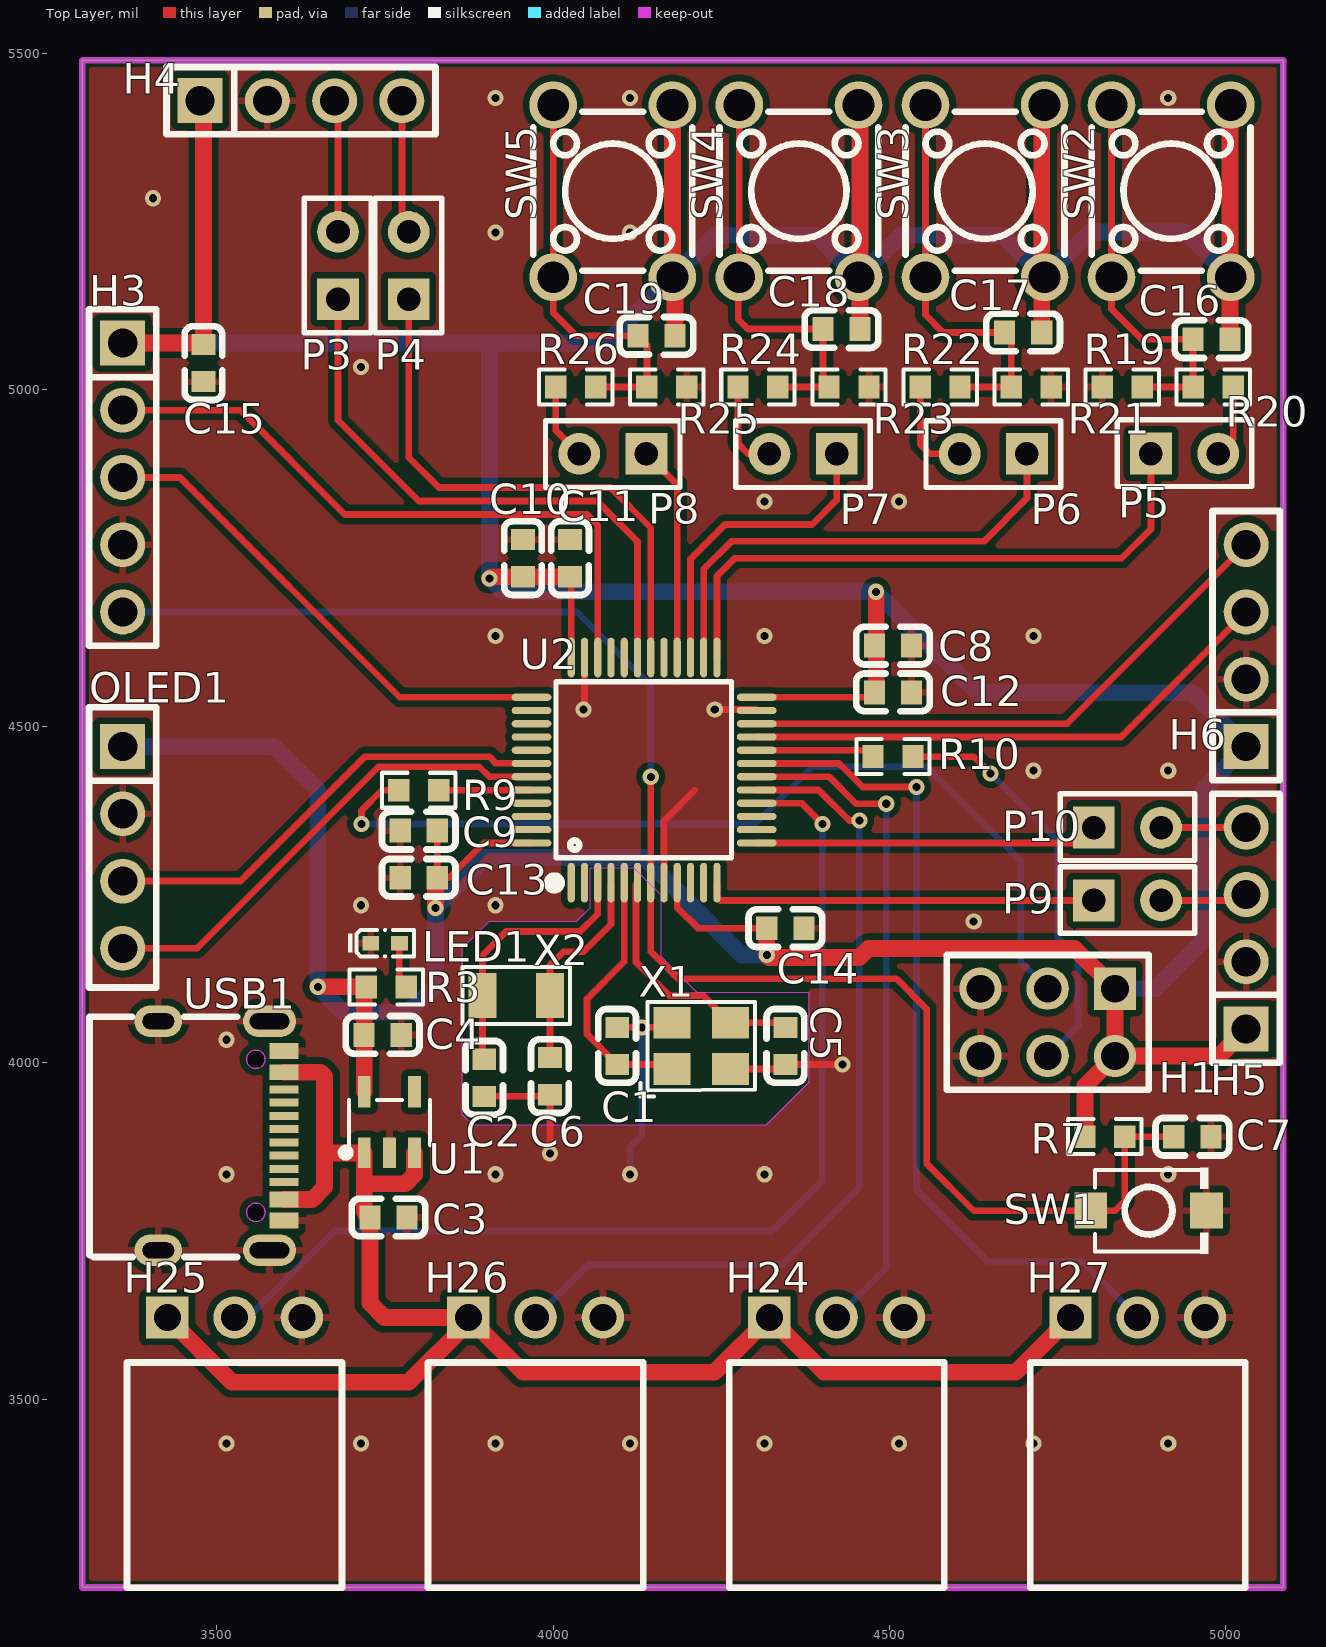
[diagram p0: Top Layer view]
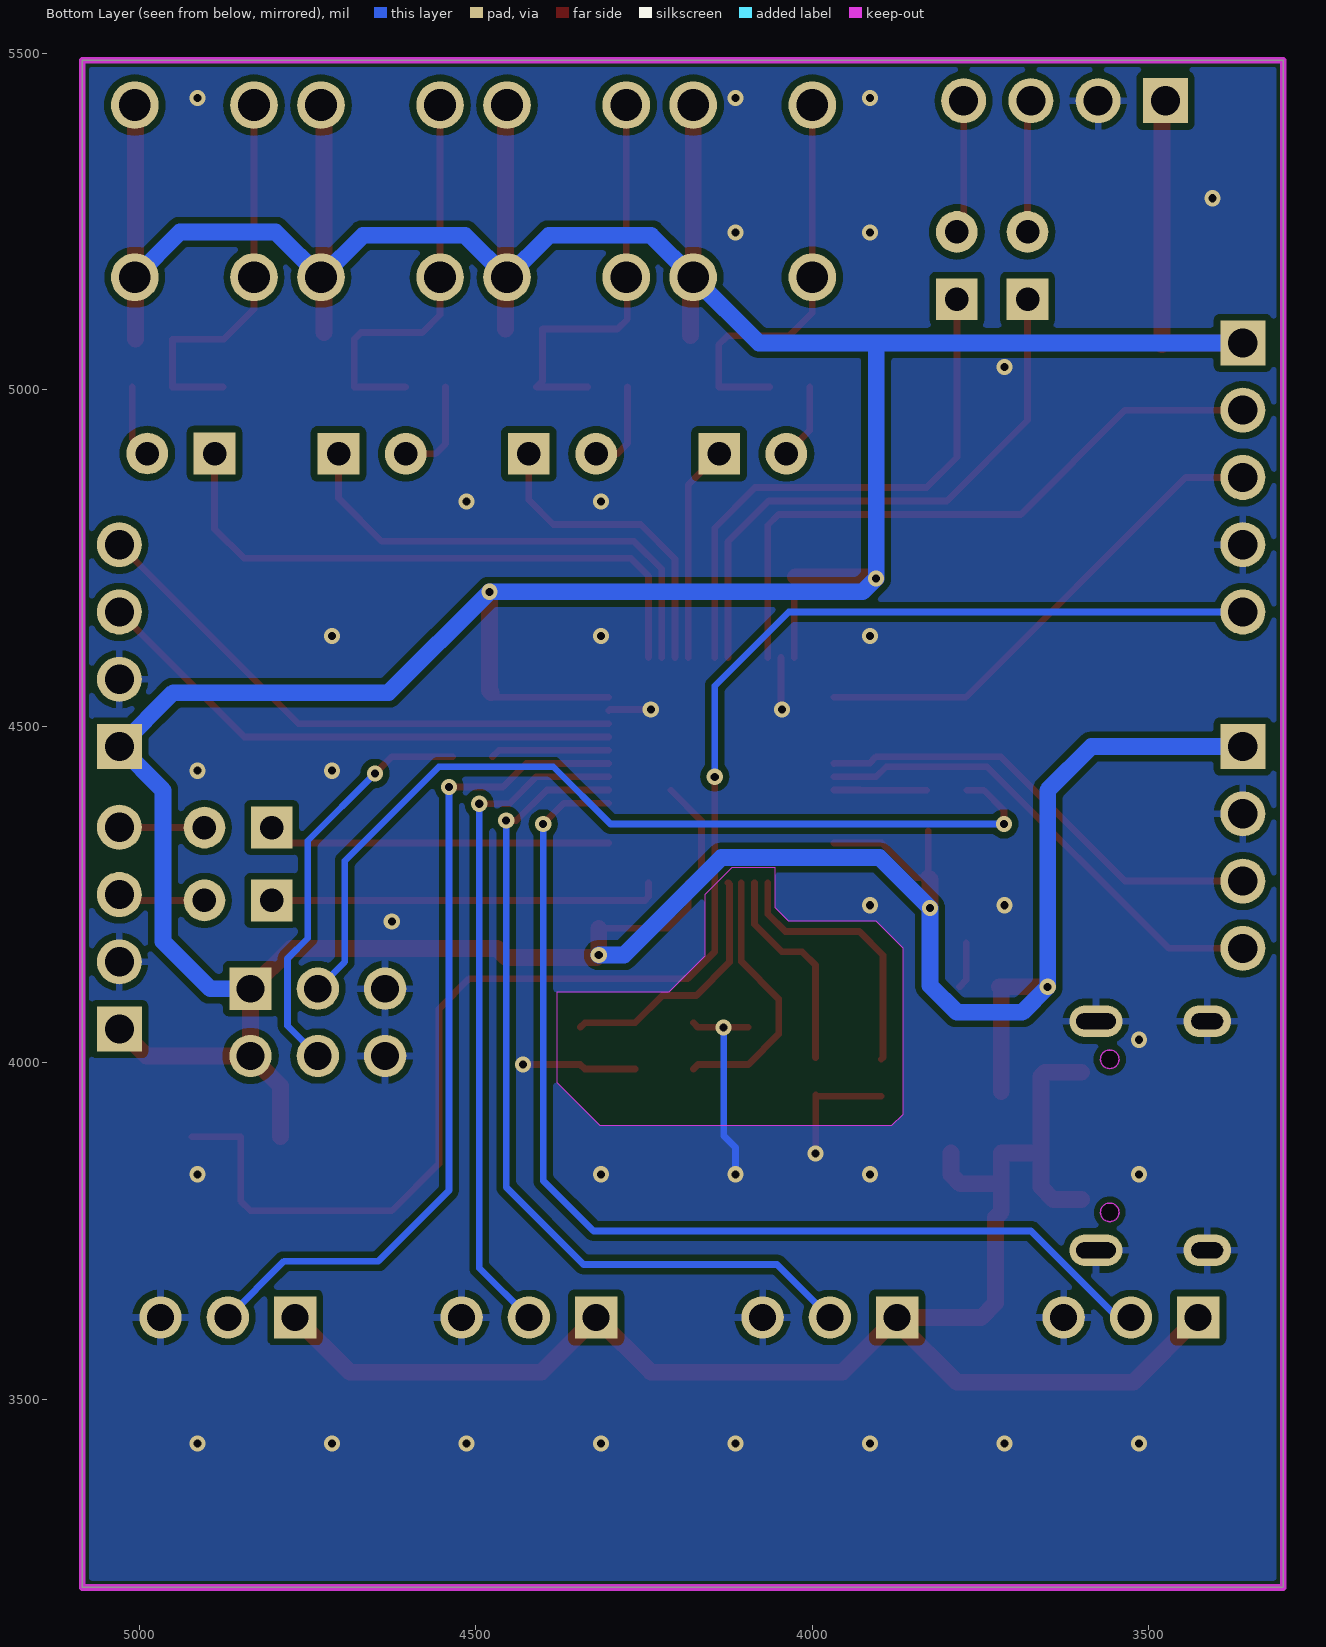
[diagram p1: Bottom Layer view, seen from below]
# Altium PCB MISC61607.pcbdoc
Units mil, origin at the board's own origin, x right, y up, seen from the top; angles counter-clockwise.
Board outline 1785 x 2270 mil, 2 copper layers (Top Layer, Bottom Layer), stack 62.206 mil thick; 60 components, 58 nets, 212 pads, 48 vias.

## Layer stack, top to bottom
Top Solder Mask Layer: solder mask 0.394, Dk 3.3
Top Layer: signal copper 1.379
Dielectric1: surface 59.449, FR4, Dk 4.5
Bottom Layer: signal copper 1.378
Bottom Solder Mask Layer: solder mask 0.394, Dk 3.3

## Board outline
3300,5490 3300,3220 5085,3220 5085,5490

## Design rules (kind name [scope] priority, off if disabled: settings)
BoardOutlineClearance copperThickness2oz_1 [All] p2 off: genericclearance=7.99 ignorepadtopadclearanceinfootprint=FALSE except(0: Arc-SplitContinuation Track-SplitContinuation SMDPad-SplitContinuation THPad-SplitContinuation Via-SplitContinuation Fill-SplitContinuation Region-SplitContinuation Poly-SplitContinuation Text-SplitContinuation Hole-SplitContinuation; 5.98: Arc-CutoutEdge SMDPad-CutoutEdge THPad-CutoutEdge Via-CutoutEdge Fill-CutoutEdge Region-CutoutEdge Text-CutoutEdge; 6.93: Hole-OutlineEdge Hole-CutoutEdge; 10: Poly-OutlineEdge Poly-CutoutEdge; 11.81: Arc-OutlineEdge Track-OutlineEdge SMDPad-OutlineEdge THPad-OutlineEdge Via-OutlineEdge Fill-OutlineEdge Region-OutlineEdge Text-OutlineEdge Track-CutoutEdge)
BoardOutlineClearance copperThickness1oz_1 [All] p4: genericclearance=4.02 ignorepadtopadclearanceinfootprint=FALSE except(0: Arc-SplitContinuation Track-SplitContinuation SMDPad-SplitContinuation THPad-SplitContinuation Via-SplitContinuation Fill-SplitContinuation Region-SplitContinuation Poly-SplitContinuation Text-SplitContinuation Hole-SplitContinuation; 6: SMDPad-CutoutEdge THPad-CutoutEdge Via-CutoutEdge Fill-CutoutEdge Region-CutoutEdge Text-CutoutEdge; 6.93: Hole-OutlineEdge Hole-CutoutEdge; 10: Poly-OutlineEdge Poly-CutoutEdge; 11.8: Arc-OutlineEdge Track-OutlineEdge SMDPad-OutlineEdge THPad-OutlineEdge Via-OutlineEdge Fill-OutlineEdge Region-OutlineEdge Text-OutlineEdge; 11.81: Arc-CutoutEdge Track-CutoutEdge)
Clearance copperThickness2oz [All] p1 off: gap=7.99 ignorepadtopadclearanceinfootprint=FALSE except(5.98: SMDPad-Track SMDPad-SMDPad THPad-Track SMDPad-THPad THPad-THPad Track-Via SMDPad-Via THPad-Via Via-Via Fill-Track Region-Track Fill-SMDPad Region-SMDPad Fill-THPad Region-THPad Fill-Via Region-Via Fill-Fill Fill-Region Region-Region Arc-Track Arc-SMDPad Arc-THPad Arc-Via Fill-Arc Region-Arc Arc-Arc Text-Track SMDPad-Text Text-THPad Text-Via Fill-Text Region-Text Arc-Text Text-Text; 6.93: Hole-Track Hole-SMDPad Hole-THPad Hole-Via Fill-Hole Region-Hole Hole-Arc Hole-Text; 10: Poly-Track Poly-SMDPad Poly-THPad Poly-Via Poly-Fill Poly-Region Poly-Poly Poly-Arc Poly-Text Poly-Hole)
Clearance copperThickness1oz [All] p3: gap=4.02 ignorepadtopadclearanceinfootprint=FALSE except(5.98: SMDPad-Track SMDPad-SMDPad THPad-Track SMDPad-THPad THPad-THPad Track-Via SMDPad-Via THPad-Via Via-Via Fill-Track Region-Track Fill-SMDPad Region-SMDPad Fill-THPad Region-THPad Fill-Via Region-Via Fill-Fill Fill-Region Region-Region; 6: Arc-Track Arc-SMDPad Arc-THPad Arc-Via Fill-Arc Region-Arc Arc-Arc Text-Track SMDPad-Text Text-THPad Text-Via Fill-Text Region-Text Arc-Text Text-Text; 6.93: Hole-Track Hole-SMDPad Hole-THPad Hole-Via Fill-Hole Region-Hole Hole-Arc Hole-Text; 10: Poly-Track Poly-SMDPad Poly-THPad Poly-Via Poly-Fill Poly-Region Poly-Poly Poly-Arc Poly-Text Poly-Hole)
DiffPairsRouting differentialPair [All] p1: maxlimit=6 minlimit=6 mostfreqgap=6 toplayer_minwidth=5 toplayer_prefwidth=10 toplayer_maxwidth=100 toplayer_mingap=6 toplayer_prefgap=6 toplayer_maxgap=6 bottomlayer_minwidth=5 bottomlayer_prefwidth=10 bottomlayer_maxwidth=100 bottomlayer_mingap=6 bottomlayer_prefgap=6 bottomlayer_maxgap=6 maxuncoupledlength=10
HoleToHoleClearance otherClearance [All] p1: gap=11.81 allowstackedmicrovias=TRUE
Length netLength [All] p1: minlimit=0 maxlimit=0
MatchedLengths netLengthTolerance [All] p1: tolerance=1000
PasteMaskExpansion pasteMaskExpansion [All] p1: expansion=0
PlaneConnect innerPlane [All] p1: planeconnectstyle=Relief reliefexpansion=20 reliefentries=4 reliefconductorwidth=10 reliefairgap=10
PolygonConnect copperRegion [(InNet('GND'))] p1: connectstyle=Relief reliefconductorwidth=10 reliefentries=4 polygonreliefangle="90 Angle" airgapwidth=10 via.connectstyle=Relief via.reliefconductorwidth=10 via.reliefentries=4 via.polygonreliefangle="90 Angle" via.airgapwidth=10
RoutingVias viaSize [All] p1: holewidth=12.01 width=24.02 viastyle="Through Hole" minholewidth=11.81 minwidth=19.68 maxholewidth=248.03 maxwidth=393.7
SolderMaskExpansion solderMaskExpansion [IsVia] p1: expansion=-1000 istentingtop=TRUE
SolderMaskExpansion solderMaskExpansion [All] p2: expansion=2 istentingtop=FALSE
Width copperThickness2oz_2 [All] p1 off: maxlimit=100 minlimit=8 preferedwidth=10
Width copperThickness1oz_2 [All] p2: maxlimit=100 minlimit=5 preferedwidth=10

## Components (designator, comment, footprint, x,y, rotation, side; value= is the part's Value field where it differs from the comment)
C1 "18pF" C0603 4095,4025 r90 top
C2 "10pF" C0603 3897.44,3977.56 r90 top
C3 "1uF" C0603 3755,3770 r180 top
C4 "1uF" C0603 3746.42,4041.36 r180 top
C5 "18pF" C0603 4345,4025 r270 top
C6 "10pF" C0603 3995,3980 r90 top
C7 "1uF" C0603 4950,3890 r0 top
C8 "4.7uF" C0603 4505,4620 r180 top
C9 "100nF" C0603 3800,4345 r180 top
C10 "100nF" C0603 3955,4750 r90 top
C11 "100nF" C0603 4025,4750 r270 top
C12 "100nF" C0603 4505,4550.53 r180 top
C13 "100nF" C0603 3800,4275 r0 top
C14 "100nF" C0603 4345,4200 r180 top
C15 "100nF" C0603 3480,5040 r90 top
C16 "100nF" C0603 4978.47,5075.55 r0 top
C17 "100nF" C0603 4698.47,5085.55 r0 top
C18 "100nF" C0603 4428.47,5090.55 r0 top
C19 "100nF" C0603 4153.47,5080.55 r0 top
H1 "" HDR-TH_6P-P2.54-V-R2-C3-S2.54_A2541WV-2X3P 4735,4060 r180 top
H3 "PZ254V-11-05P" HDR-TH_5P-P2.54-V-M 3360,4870 r270 top
H4 "PZ254V-11-04P" HDR-TH_4P-P2.54-V-M 3625,5430 r0 top
H5 "PZ254V-11-04P" HDR-TH_4P-P2.54-V-M 5030,4200 r90 top
H6 "PZ254V-11-04P" HDR-TH_4P-P2.54-V-M 5030,4620 r90 top
H24 "HC-PM254-8.5H-1x3PW-02A" HDR-TH_3P-P2.54_HC-PM254-8.5H-1X3PW 4421.3,3621.27 r0 top
H25 "HC-PM254-8.5H-1x3PW-02A" HDR-TH_3P-P2.54_HC-PM254-8.5H-1X3PW 3526.27,3621.27 r0 top
H26 "HC-PM254-8.5H-1x3PW-02A" HDR-TH_3P-P2.54_HC-PM254-8.5H-1X3PW 3973.78,3621.27 r0 top
H27 "HC-PM254-8.5H-1x3PW-02A" HDR-TH_3P-P2.54_HC-PM254-8.5H-1X3PW 4868.81,3621.27 r0 top
LED1 "" LED_0402 3749.97,4177.82 r0 top
OLED1 "2.54-1*4P female" HDR-TH_4P-P2.54-V-F 3360,4320 r270 top
P3 "Jumper pin header" 2P排针 3680,5185 r90 top
P4 "Jumper pin header" 2P排针 3785,5185 r90 top
P5 "Jumper pin header" 2P排针 4938.47,4905.55 r0 top
P6 "Jumper pin header" 2P排针 4654.16,4905.08 r180 top
P7 "Jumper pin header" 2P排针 4371.31,4905.08 r180 top
P8 "Jumper pin header" 2P排针 4088.47,4905.08 r180 top
P9 "Jumper pin header" 2P排针 4853.54,4241.28 r0 top
P10 "Jumper pin header" 2P排针 4853.54,4349.54 r0 top
R3 "1kΩ" R0603 3751.58,4112.82 r0 top
R7 "10kΩ" R0603 4820,3890 r180 top
R9 "10kΩ" R0603 3800,4405 r180 top
R10 "10kΩ" R0603 4505,4455 r180 top
R19 "4.7kΩ" R0603 4845.78,5004.36 r0 top
R20 "1kΩ" R0603 4981.17,5004.36 r180 top
R21 "4.7kΩ" R0603 4710.4,5004.36 r180 top
R22 "1kΩ" R0603 4575.01,5004.36 r0 top
R23 "4.7kΩ" R0603 4439.62,5004.36 r180 top
R24 "1kΩ" R0603 4304.24,5004.36 r0 top
R25 "4.7kΩ" R0603 4168.85,5004.36 r180 top
R26 "1kΩ" R0603 4033.47,5004.36 r0 top
SW1 "TS-1088-AR02016" SW-SMD_L3.9-W3.0-P4.45 4885,3780 r0 top
SW2 "TS665CJ" SW-TH_4P-L6.0-W6.0-P4.50-LS6.5 4918.47,5295.55 r90 top
SW3 "TS665CJ" SW-TH_4P-L6.0-W6.0-P4.50-LS6.5 4641.8,5295.55 r90 top
SW4 "TS665CJ" SW-TH_4P-L6.0-W6.0-P4.50-LS6.5 4365.13,5295.55 r90 top
SW5 "TS665CJ" SW-TH_4P-L6.0-W6.0-P4.50-LS6.5 4088.47,5295.55 r90 top
U1 "ME6211C33M5G-N" SOT-23-5_L3.0-W1.7-P0.95-LS2.8-BL 3756.42,3911.36 r0 top
U2 "STM32F103C8T6" LQFP-48_L7.0-W7.0-P0.50-LS9.0-BL 4135,4435 r0 top
USB1 "TYPE-C 16PIN 2MD(073)" USB-C-SMD_TYPE-C-6PIN-2MD-073 3506.42,3891.36 r270 top
X1 "8MHz" OSC-SMD_4P-L3.2-W2.5-BL 4220,4025 r0 top
X2 "32.768kHz" CRYSTAL-SMD_L3.2-W1.5-1 3945,4100 r180 top

## Footprints (in the part's own frame and the unit in brackets; to place one, negate y for a bottom-side part, rotate by r counter-clockwise, add the part's x,y. Pads: shape width x height; smd on the part's side, far side on the other; paste and mask are expansions set on the pad)
2P排针 [mil]
  rect 62x62 hole 35: 1(-50,0)
  round 62 hole 35: 2(50,0)
  silkscreen extent -100,-49 100,50
C0603 [mm]
  rect 0.8x0.9 smd: 1(-0.7,0) 2(0.7,0)
  silkscreen extent -1.39,-0.71 1.39,0.71
CRYSTAL-SMD_L3.2-W1.5-1 [mm]
  rect 1.05x1.7 smd: 1(-1.275,0) 2(1.275,0)
  silkscreen extent -2.03,-1.08 2.03,1.08
HDR-TH_3P-P2.54_HC-PM254-8.5H-1X3PW [mm]
  rect 1.6x1.6 hole 1.02: 1(-2.54,0)
  round 1.6 hole 1.02: 2(0,0) 3(2.54,0)
  silkscreen extent -4.06,-10.2 4.06,-1.7
HDR-TH_4P-P2.54-V-F [mm]
  rect 1.7x1.7 hole 1.1: 1(-3.81,0)
  round 1.7 hole 1.1: 2(-1.27,0) 3(1.27,0) 4(3.81,0)
  silkscreen extent -5.29,-1.27 5.29,1.27
HDR-TH_4P-P2.54-V-M [mm]
  rect 1.7x1.7 hole 1.1: 1(-3.81,0)
  round 1.7 hole 1.1: 2(-1.27,0) 3(1.27,0) 4(3.81,0)
  silkscreen extent -5.08,-1.27 5.08,1.27
HDR-TH_5P-P2.54-V-M [mm]
  rect 1.7x1.7 hole 1.1: 1(-5.08,0)
  round 1.7 hole 1.1: 2(-2.54,0) 3(0,0) 4(2.54,0) 5(5.08,0)
  silkscreen extent -6.35,-1.27 6.35,1.27
HDR-TH_6P-P2.54-V-R2-C3-S2.54_A2541WV-2X3P [mm]
  rect 1.6x1.6 hole 1.05: 1(-2.54,-1.27)
  round 1.6 hole 1.05: 2(-2.54,1.27) 3(0,-1.27) 4(0,1.27) 5(2.54,-1.27) 6(2.54,1.27)
  silkscreen extent -3.81,-2.54 3.81,2.54
LED_0402 [mil]
  rect 25.1x21.3 smd paste-3937.01 mask+2: 1(-21.2,0) 2(21.2,0)
  silkscreen extent -55,-21 43,21
LQFP-48_L7.0-W7.0-P0.50-LS9.0-BL [mm]
  oval 0.27x1.5 smd paste+0 mask+0.05: 1(-2.75,-4.25) 2(-2.25,-4.25) 3(-1.75,-4.25) 4(-1.25,-4.25) 5(-0.75,-4.25) 6(-0.25,-4.25) 7(0.25,-4.25) 8(0.75,-4.25) 9(1.25,-4.25) 10(1.75,-4.25) 11(2.25,-4.25) 12(2.75,-4.25) 25(2.75,4.25) 26(2.25,4.25) 27(1.75,4.25) 28(1.25,4.25) 29(0.75,4.25) 30(0.25,4.25) 31(-0.25,4.25) 32(-0.75,4.25) 33(-1.25,4.25) 34(-1.75,4.25) 35(-2.25,4.25) 36(-2.75,4.25)
  oval 1.5x0.27 smd paste+0 mask+0.05: 13(4.25,-2.75) 14(4.25,-2.25) 15(4.25,-1.75) 16(4.25,-1.25) 17(4.25,-0.75) 18(4.25,-0.25) 19(4.25,0.25) 20(4.25,0.75) 21(4.25,1.25) 22(4.25,1.75) 23(4.25,2.25) 24(4.25,2.75) 37(-4.25,2.75) 38(-4.25,2.25) 39(-4.25,1.75) 40(-4.25,1.25) 41(-4.25,0.75) 42(-4.25,0.25) 43(-4.25,-0.25) 44(-4.25,-0.75) 45(-4.25,-1.25) 46(-4.25,-1.75) 47(-4.25,-2.25) 48(-4.25,-2.75)
  silkscreen extent -3.59,-4.46 3.3,3.34
OSC-SMD_4P-L3.2-W2.5-BL [mm]
  rect 1.4x1.2 smd: 1(-1.1,-0.875) 2(1.1,-0.875) 3(1.1,0.875) 4(-1.1,0.875)
  silkscreen extent -2.29,-1.9 2.03,1.65
R0603 [mil]
  rect 31.75x34.02 smd paste-3937.01 mask+2: 1(-29.66,0) 2(29.66,0)
  silkscreen extent -55,-26 55,26
SOT-23-5_L3.0-W1.7-P0.95-LS2.8-BL [mm]
  rect 0.49x1.157 smd: 1(-0.95,-1.154) 2(0,-1.154) 3(0.95,-1.154)
  rect 0.49x1.175 smd: 4(0.95,1.154) 5(-0.95,1.154)
  silkscreen extent -1.8,-1.29 1.53,0.85
SW-SMD_L3.9-W3.0-P4.45 [mm]
  rect 1.23x1.36 smd: 1(-2.185,0) 2(2.185,0)
  silkscreen extent -2.03,-1.62 2.25,1.62
SW-TH_4P-L6.0-W6.0-P4.50-LS6.5 [mm]
  round 1.8 hole 1.2: 1(-3.25,2.25) 2(3.25,2.25) 3(-3.25,-2.25) 4(3.25,-2.25)
  silkscreen extent -3,-3 3,3
USB-C-SMD_TYPE-C-6PIN-2MD-073 [mm]
  rect 0.6x1.1 smd paste-100 mask+0.05: 1(-3.2,2.375) 2(-2.4,2.375) 11(2.4,2.375) 12(3.2,2.375)
  rect 0.3x1.1 smd paste-100 mask+0.05: 3(-1.75,2.375) 4(-1.25,2.375) 5(-0.75,2.375) 6(-0.25,2.375) 7(0.25,2.375) 8(0.75,2.375) 9(1.25,2.375) 10(1.75,2.375)
  oval 1.2x2 hole 0.6 slot 1.5 at 90 deg paste+0 mask+0.05: 13(-4.325,1.825) 14(4.325,1.825)
  oval 1.2x1.8 hole 0.6 slot 1.2 at 90 deg paste+0 mask+0.05: 13(-4.325,-2.375) 14(4.325,-2.375)
  Board Outline Layer circle w0.003: c-2.89,1.305 r0.35
  Board Outline Layer circle w0.003: c2.89,1.305 r0.35
  Board Outline Layer region: -2.89,1.655 -2.738,1.62 -2.616,1.523 -2.549,1.383 -2.549,1.227 -2.616,1.087 -2.738,0.99 -2.89,0.955 -2.89,0.955 -3.042,0.99 -3.164,1.087 -3.231,1.227 -3.231,1.383 -3.164,1.523 -3.042,1.62 -2.89,1.655
  Board Outline Layer region: -2.89,1.655 -2.812,1.646 -2.738,1.62 -2.672,1.579 -2.616,1.523 -2.575,1.457 -2.549,1.383 -2.54,1.305 -2.549,1.227 -2.575,1.153 -2.616,1.087 -2.672,1.031 -2.738,0.99 -2.812,0.964 -2.89,0.955 -2.968,0.964 -3.042,0.99 -3.108,1.031 -3.164,1.087 -3.205,1.153 -3.231,1.227 -3.24,1.305 -3.231,1.383 -3.205,1.457 -3.164,1.523 -3.108,1.579 -3.042,1.62 -2.968,1.646
  Board Outline Layer region: 2.89,1.655 3.042,1.62 3.164,1.523 3.231,1.383 3.231,1.227 3.164,1.087 3.042,0.99 2.89,0.955 2.89,0.955 2.738,0.99 2.616,1.087 2.549,1.227 2.549,1.383 2.616,1.523 2.738,1.62 2.89,1.655
  Board Outline Layer region: 2.89,1.655 2.968,1.646 3.042,1.62 3.108,1.579 3.164,1.523 3.205,1.457 3.231,1.383 3.24,1.305 3.231,1.227 3.205,1.153 3.164,1.087 3.108,1.031 3.042,0.99 2.968,0.964 2.89,0.955 2.812,0.964 2.738,0.99 2.672,1.031 2.616,1.087 2.575,1.153 2.549,1.227 2.54,1.305 2.549,1.383 2.575,1.457 2.616,1.523 2.672,1.579 2.738,1.62 2.812,1.646
  Multi-Layer board cut-out: -2.89,1.655 -2.738,1.62 -2.616,1.523 -2.549,1.383 -2.549,1.227 -2.616,1.087 -2.738,0.99 -2.89,0.955 -2.89,0.955 -3.042,0.99 -3.164,1.087 -3.231,1.227 -3.231,1.383 -3.164,1.523 -3.042,1.62 -2.89,1.655
  Multi-Layer board cut-out: 2.89,1.655 3.042,1.62 3.164,1.523 3.231,1.383 3.231,1.227 3.164,1.087 3.042,0.99 2.89,0.955 2.89,0.955 2.738,0.99 2.616,1.087 2.549,1.227 2.549,1.383 2.616,1.523 2.738,1.62 2.89,1.655
  silkscreen extent -4.5,-4.97 4.57,0.6

## Via types
v1: diameter 24.02, hole 12, Top Layer to Bottom Layer, 48 vias

## Nets (pads, with @x,y where several pads share a name; then routed paths per layer and width w, separated by ;. In a path a pad name is that pad's centre, name@x,y a point inside that pad or via, vN(x,y) a via of type N, cw(c..) or ccw(c..) an arc to the next point about the centre after c; other vN are vias at no path point)
$1N5475: LED1.2 R3.2 | length 69.2
  Top Layer w10: LED1.2 3771.17,4122.88 R3.2
$1N5490: H1.4 R10.1 | length 618.2
  Top Layer w10: R10.1 4625,4455 v1(4650,4430)
  Bottom Layer w10: v1(4650,4430) 4750,4330 4750,4185 4780,4155 4780,4055 H1.4
$1N5491: H1.3 R9.2 | length 1367.5
  Top Layer w10: v1(3715,4355) 3715,4375 3745,4405 R9.2
  Bottom Layer w10: v1(3715,4355) 4300,4355 4385,4440 4555,4440 4695,4300 4695,4150 H1.3
$1N5608: H4.3 P3.2 | length 197.1
  Top Layer w10: H4.3 3680,5425 P3.2
$1N5609: H4.4 P4.2 | length 199.1
  Top Layer w10: H4.4 3775,5245 P4.2
$1N5610: C19.1 R25.2 R26.2 SW5.1 SW5.2 | length 606.5
  Top Layer w10: SW5.2 SW5.1 3999.89,5115.11 4034.45,5080.55 C19.1 4139.19,5067.26 R25.2 R26.2
$1N5614: P6.2 R22.1 | length 149.3
  Top Layer w10: R22.1 4545.35,4920 4560.26,4905.09 P6.2
$1N5615: P8.2 R26.1 | length 113.6
  Top Layer w10: R26.1 4003.81,4939.74 P8.2
$1N5618: C17.1 R21.2 R22.2 SW3.1 SW3.2 | length 601.6
  Top Layer w10: SW3.2 SW3.1 4553.22,5111.78 4579.45,5085.55 C17.1 4680.74,5075.72 R21.2 R22.2
$1N5623: P7.2 R24.1 | length 137
  Top Layer w10: R24.1 4274.58,4920.42 4289.91,4905.09 P7.2
$1N5624: C18.1 R23.2 R24.2 SW4.1 SW4.2 | length 617
  Top Layer w10: SW4.2@4276.55,5423.5 4276.55,5167.6 4275,5166.04 4275,5105 4289.45,5090.55 C18.1 4400.91,5013.42 R23.2 R24.2
$1N5632: C16.1 R19.2 R20.2 SW2.1 SW2.2 | length 590.4
  Top Layer w10: SW2.2 SW2.1 4829.89,5120.11 4874.45,5075.55 C16.1 4950.91,5004.96 R20.2 R19.2
$1N5633: P5.2 R20.1 | length 108.1
  Top Layer w10: P5.2 5010.83,4927.9 R20.1
$1N5806: H5.3 P9.2 | length 130.1
  Top Layer w10: P9.2 5021.28,4241.28 H5.3
$1N5807: H5.4 P10.2 | length 126.7
  Top Layer w10: P10.2 5029.53,4349.53 H5.4
+5V: C3.2 H24.1 H25.1 H26.1 H27.1 U1.1 U1.3 USB1.2 USB1.11 | length 2410.4
  Top Layer w25: H25.1 3522.54,3525 3785,3525 3873.78,3613.78 H26.1 ; USB1.11 3641.86,3796.86 3660,3815 3660,3865.94 ; USB1.2 3654.16,3985.84 3660,3980 3660,3865.94 ; U1.3 3793.82,3833.82 3780,3820 3719.74,3820 3719.02,3819.28 ; H27.1 4687.54,3540 4402.57,3540 H24.1 4240.03,3540 3955.05,3540 H26.1 ; 3660,3865.94 U1.1 3719.02,3819.28 ; 3719.02,3819.28 3719.02,3778.42 C3.2 3727.44,3642.56 3748.73,3621.27 H26.1
BOOT0: R9.1 U2.44 | length 138.2
  Top Layer w10: R9.1 3929.06,4405 3929.53,4405.47 U2.44
BOOT1: R10.2 U2.20 | length 177
  Top Layer w10: U2.20 4465.81,4464.53 R10.2
GND: C1.2 C2.1 C3.1 C4.1 C5.2 C6.1 C7.2 C8.1 C9.2 C10.2 C11.1 C12.1 C13.1 C14.1 C15.1 H1.5 H1.6 H3.4 H4.2 H5.2 H6.2 H24.3 H25.3 H26.3 H27.3 LED1.1 OLED1.2 R19.1 R21.1 R23.1 R25.1 SW1.2 U1.2 U2.8 U2.23 U2.35 USB1.1 USB1.12 USB1.13 USB1.14 X1.2 X1.4 | length 962.8
  Top Layer w10: C2.1 3992.56,3950 C6.1 v1(3995,3865) ; v1(4045,4525) 4046.42,4526.42 U2.35 ; C1.2 v1(4131.72,4052.56) 4169.8,4052.56 X1.4 ; U2.8 4164.53,4359.53 4210,4405 ; v1(4240,4525) 4300.9,4525 U2.23 ; X1.2 4338.11,3990.55 C5.2 v1(4430,3997.44)
  Bottom Layer w10: v1(4114.1,3834.1) 4114.1,3874.1 4131.72,3891.72 v1(4131.72,4052.56)
  other v1: 3514.1,3434.1 3714.1,3434.1 3914.1,3434.1 4114.1,3434.1 4314.1,3434.1 4514.1,3434.1 4714.1,3434.1 4914.1,3434.1 3514.1,3834.1 3914.1,3834.1 4314.1,3834.1 4914.1,3834.1 3514.1,4034.1 4625,4210 3714.1,4234.1 3914.1,4234.1 4714.1,4434.1 4914.1,4434.1 3914.1,4634.1 4314.1,4634.1 4714.1,4634.1 4314.1,4834.1 4514.1,4834.1 3714.1,5034.1 3914.1,5234.1 4114.1,5234.1 3405,5285 3914.1,5434.1 4114.1,5434.1 4914.1,5434.1
NRST: C7.1 H3.5 R7.1 SW1.1 U2.7 | length 2398.8
  Top Layer w10: v1(4145,4425) 4145,4267.84 U2.7 4144.84,4165.16 4185,4125 4510,4125 4555,4080 4555,3850 4625,3780 SW1.1 4835,3780 4849.66,3794.66 R7.1 C7.1
  Bottom Layer w10: H3.5 4035,4670 4145,4560 v1(4145,4425)
OSC32_IN: C2.2 U2.3 X2.2 | length 399
  Top Layer w10: C2.2 3894.81,4007.75 X2.2 3894.81,4159.81 3930,4195 4040,4195 4066.1,4221.1 U2.3
OSC32_OUT: C6.2 U2.4 X2.1 | length 315.3
  Top Layer w10: C6.2 3995.2,4007.76 X2.1 3995.2,4145.2 4015,4165 4045,4165 4085.79,4205.79 U2.4
OSC_IN: C1.1 U2.5 X1.1 | length 396.4
  Top Layer w10: U2.5 4105.47,4150.47 4050,4095 4050,4042.44 C1.1 4169.8,3997.44 X1.1
OSC_OUT: C5.1 U2.6 X1.3 | length 381.4
  Top Layer w10: U2.6 4122.93,4265.45 4122.93,4149.43 4172.36,4100 4222.76,4100 X1.3 4338.11,4059.45 C5.1
PA0: U2.10
PA1: U2.11
PA2: P9.1 U2.12 | length 583.5
  Top Layer w10: U2.12 4243.27,4246.73 4248.72,4241.28 P9.1
PA3: P10.1 U2.13 | length 510.7
  Top Layer w10: U2.13 4780.74,4326.73 P10.1
PA4: U2.14
PA5: U2.15
PA6: H25.2 U2.16 | length 1598.6
  Top Layer w10: U2.16 4369.21,4385.79 v1(4400,4355)
  Bottom Layer w10: H25.2 3546.27,3621.27 3675,3750 4325,3750 4400,3825 v1(4400,4355)
PA7: H26.2 U2.17 | length 1278
  Top Layer w10: U2.17 4394.53,4405.47 4440,4360 v1(4455,4360)
  Bottom Layer w10: H26.2 4052.52,3700 4340,3700 4455,3815 v1(4455,4360)
PA8: U2.29
PA9: P4.1 U2.30 | length 831.1
  Top Layer w10: P4.1 3785,4900 3830,4855 4085,4855 4144.84,4795.16 U2.30
PA10: P3.1 U2.31 | length 872.3
  Top Layer w10: P3.1 3680,4955 3800,4835 4065,4835 4125.16,4774.84 U2.31
PA11: U2.32
PA12: U2.33
PA13: H3.2 U2.34 | length 973.6
  Top Layer w10: H3.2 3535,4970 3690,4815 4050,4815 4066.1,4798.9 U2.34
PA14: H3.3 U2.37 | length 743
  Top Layer w10: H3.3 3445,4870 3771.73,4543.27 U2.37
PA15: U2.38
PB0: H24.2 U2.18 | length 1003.6
  Top Layer w10: U2.18 4409.84,4425.16 4450,4385 v1(4495,4385)
  Bottom Layer w10: H24.2 4495,3694.97 v1(4495,4385)
PB1: H27.2 U2.19 | length 1259.1
  Top Layer w10: U2.19 4425.16,4444.84 4460,4410 v1(4540,4410)
  Bottom Layer w10: v1(4540,4410) 4540,3810 4645,3705 4785.08,3705 H27.2
PB3: U2.39
PB4: U2.40
PB5: U2.41
PB6: OLED1.3 U2.42 | length 688.5
  Top Layer w10: OLED1.3 3535,4270 3720,4455 3905,4455 3915,4445 3967.52,4445 U2.42
PB7: OLED1.4 U2.43 | length 725.7
  Top Layer w10: OLED1.4 3470,4170 3740,4440 3890,4440 3904.84,4425.16 U2.43
PB8: U2.45
PB9: U2.46
PB10: H6.3 U2.21 | length 804.6
  Top Layer w10: U2.21 4844.21,4484.21 H6.3
PB11: H6.4 U2.22 | length 837.9
  Top Layer w10: U2.22 4763.9,4503.9 H6.4
PB12: P5.1 U2.25 | length 907.3
  Top Layer w10: U2.25 4243.27,4723.27 4270,4750 4845,4750 4888.47,4793.47 P5.1
PB13: P6.1 U2.26 | length 721.5
  Top Layer w10: U2.26 4223.58,4733.58 4265,4775 4640,4775 4704.16,4839.16 P6.1
PB14: P7.1 U2.27 | length 469
  Top Layer w10: U2.27 4203.9,4748.9 4255,4800 4385,4800 4421.31,4836.31 P7.1
PB15: P8.1 U2.28 | length 321.7
  Top Layer w10: P8.1 4184.21,4859.34 U2.28
PC13: U2.2
VBAT: U2.1
VCC: C4.2 C8.2 C9.1 C10.1 C11.2 C12.2 C13.2 C14.2 C15.2 C16.2 C17.2 C18.2 C19.2 H1.1 H1.2 H3.1 H4.1 H5.1 H6.1 OLED1.1 R3.1 R7.2 SW2.3 SW2.4 SW3.3 SW3.4 SW4.3 SW4.4 SW5.3 SW5.4 U1.5 U2.9 U2.24 U2.36 U2.48 | length 9568.1
  Top Layer w10: C9.1 C13.2 3845,4275 3896.73,4326.73 U2.48 ; C11.2 4026.73,4720.71 U2.36 ; U2.9 4184.21,4230.79 4215,4200 C14.2 ; U2.24 4470.18,4543.27 C12.2
  Top Layer w25: H3.1 3477.56,5070 C15.2 3480,5425 H4.1 ; v1(3650,4112.82) R3.1 3719.02,4109.92 U1.5 ; v1(3825,4230) 3825,4272.44 C13.2 ; v1(3905,4720) 3907.44,4722.44 C10.1 C11.2 ; SW5.4 SW5.3 4181.03,5163.62 C19.2 ; C14.2 v1(4317.44,4160) 4320.92,4156.52 4455,4156.52 4468.48,4170 4775,4170 H1.1 H1.2 ; SW4.4 4456.03,5421.18 C18.2 ; C12.2 4480,4553.09 v1(4480,4700) ; C17.2 4726.03,5419.14 SW3.4 ; R7.2 4790.34,3965.34 H1.2 ; C16.2 5006.03,5422.48 SW2.4 ; H5.1 4990,4010 H1.2
  Bottom Layer w25: OLED1.1 3585,4470 3650,4405 v1(3650,4112.82) 3687.82,4075 3785,4075 3825,4115 v1(3825,4230) 3900,4305 4135,4305 4280,4160 v1(4317.44,4160) ; H3.1 3904.47,5070 ; H1.1 4895,4110 4965,4180 4965,4405 H6.1 4950,4550 4630,4550 v1(4480,4700) 3925,4700 v1(3905,4720) 3905,5069.47 3904.47,5070 ; SW2.3 4939.64,5235 4797.78,5235 SW3.3 4667.98,5230 4516.12,5230 SW4.3 4391.31,5230 4239.45,5230 SW5.3 4079.45,5070 3904.47,5070
pads on no net: U1.4 U2.47 USB1.3 USB1.4 USB1.5 USB1.6 USB1.7 USB1.8 USB1.9 USB1.10

## Polygon pours and split planes (outlines as drawn)
GND on Bottom Layer (solid, remove dead copper, pour order 2): 3000,5690 3000,3000 5470,3000 5470,5690
GND on Top Layer (solid, remove dead copper, pour order 0): 3175,5615 3175,3035 5415,3035 5415,5615

## Keep-outs
Board Outline Layer:
  region: 4055,4290 4120,4290 4160,4250 4160,4158.16 4213.16,4105 4380,4105 4380,3970.99 4315.93,3906.92 3881.68,3906.92 3865,3923.6 3865,4170 3905,4210 4035,4210 4055,4230
  lines w10: 3300,3220 3300,5490 5085,5490 5085,3220 3300,3220